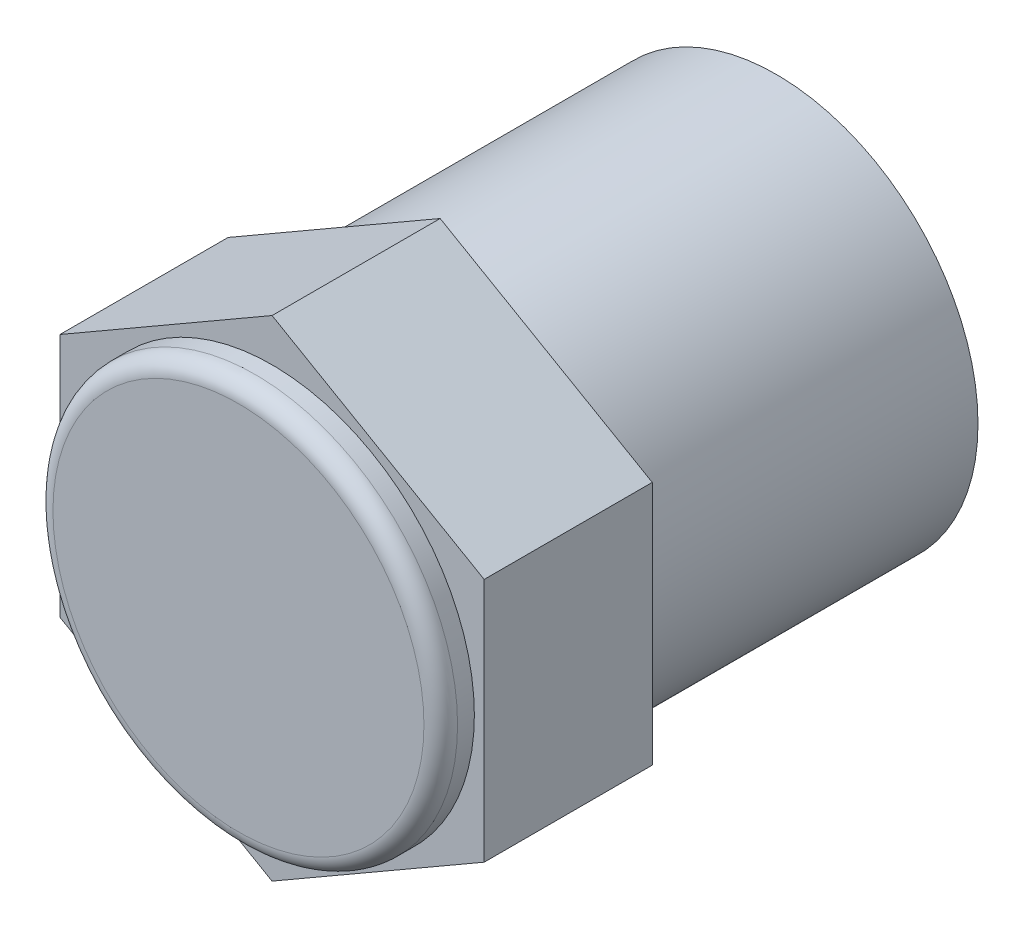
from build123d import *

# Parameters (mm, degrees)
SKETCH1_R           = 6
BOSS_EXTRUDE1_DEPTH = 10
BOSS_EXTRUDE2_DEPTH = 5
SKETCH3_R           = 6.018032789
BOSS_EXTRUDE3_DEPTH = 1
FILLET2_R           = 0.5


with BuildPart() as part:
    # Sketch1 → Boss-Extrude1 (new body)
    with BuildSketch(Plane.XY):
        Circle(SKETCH1_R)
    extrude(amount=BOSS_EXTRUDE1_DEPTH)

    # Sketch2 → Boss-Extrude2 (add)
    with BuildSketch(Plane.XY.offset(10)):
        Polygon((0, 7.285798141), (-6.309686277, 3.64289907), (-6.309686277, -3.64289907), (0, -7.285798141), (6.309686277, -3.64289907), (6.309686277, 3.64289907), align=None)
    extrude(amount=BOSS_EXTRUDE2_DEPTH)

    # Sketch3 → Boss-Extrude3 (add)
    with BuildSketch(Plane.XY.offset(15)):
        Circle(SKETCH3_R)
    extrude(amount=BOSS_EXTRUDE3_DEPTH)

    # Fillet2
    fillet2_edges = [part.edges().sort_by_distance(p)[0] for p in [
        (-6.018032789, 0, 16),
    ]]
    fillet(fillet2_edges, radius=FILLET2_R)


solid = part.part
